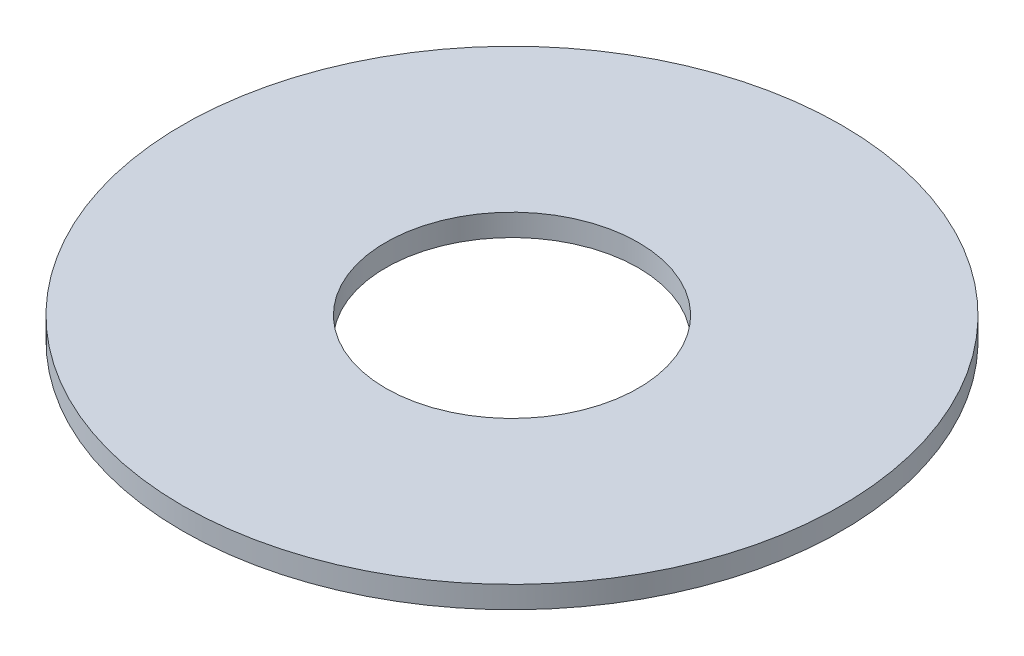
from build123d import *

# Parameters (mm, degrees)
SKETCH1_R           = 30
SKETCH1_R_2         = 11.5
BOSS_EXTRUDE1_DEPTH = 2


with BuildPart() as part:
    # Sketch1 → Boss-Extrude1 (new body)
    with BuildSketch(Plane(origin=(0, 0, 0), x_dir=(1, 0, 0), z_dir=(0, 1, 0))):
        with Locations(Location((0, 0, 0), (0, 0, 270))):
            Circle(SKETCH1_R)
        with Locations(Location((0, 0, 0), (0, 0, 270))):
            Circle(SKETCH1_R_2, mode=Mode.SUBTRACT)
    extrude(amount=BOSS_EXTRUDE1_DEPTH)


solid = part.part
